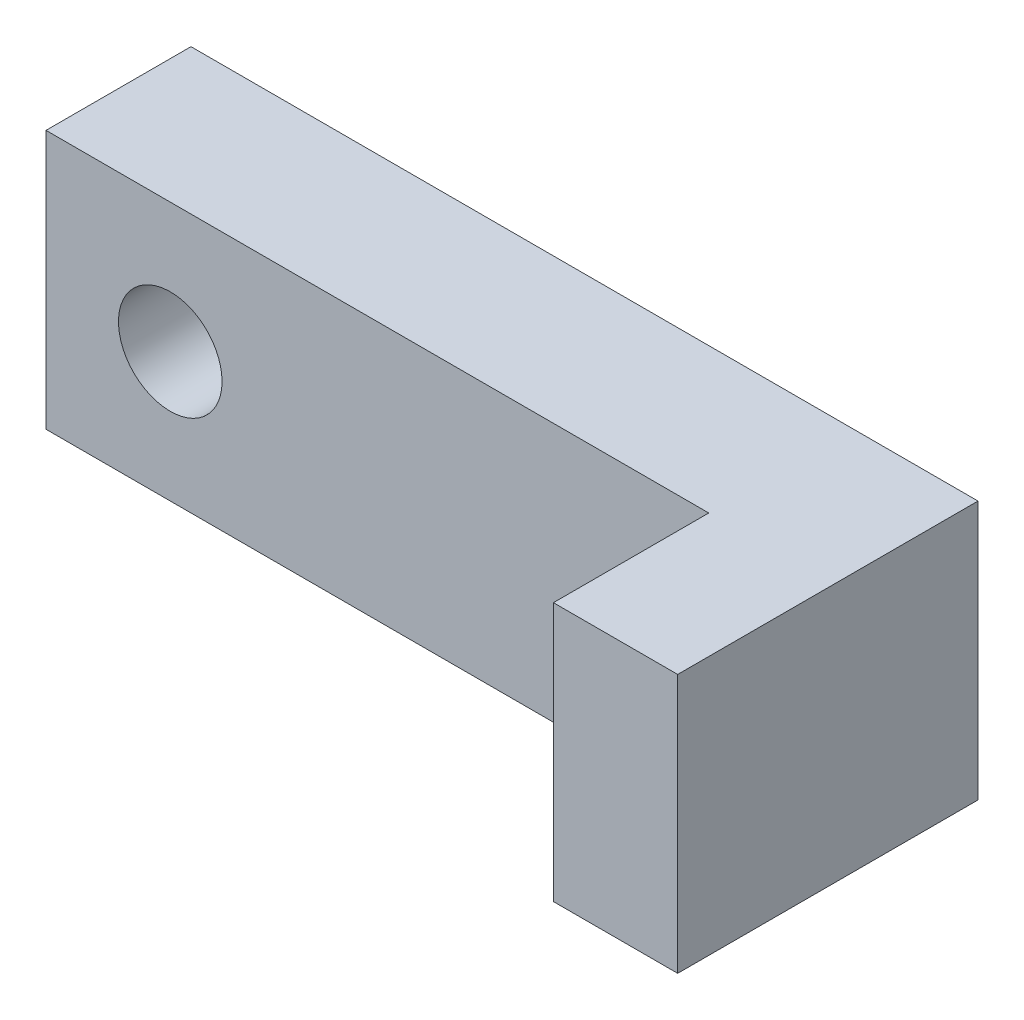
from build123d import *

# Parameters (mm, degrees)
SKETCH_1_W      = 76
SKETCH_1_H      = 25
SKETCH_1_R      = 5
EXTRUDE_1_DEPTH = 7
SKETCH_2_W      = 12
SKETCH_2_H      = 25
EXTRUDE_2_DEPTH = 15


with BuildPart() as part:
    # 草图1 → 凸台-拉伸1 (new, symmetric)
    with BuildSketch(Plane.XY):
        Rectangle(SKETCH_1_W, SKETCH_1_H)
        with Locations((-26, 0)):
            Circle(SKETCH_1_R, mode=Mode.SUBTRACT)
    extrude(amount=EXTRUDE_1_DEPTH, both=True)

    # 草图2 → 凸台-拉伸2 (add)
    with BuildSketch(Plane.XY.offset(7)):
        with Locations((32, 0)):
            Rectangle(SKETCH_2_W, SKETCH_2_H)
    extrude(amount=EXTRUDE_2_DEPTH)


solid = part.part
